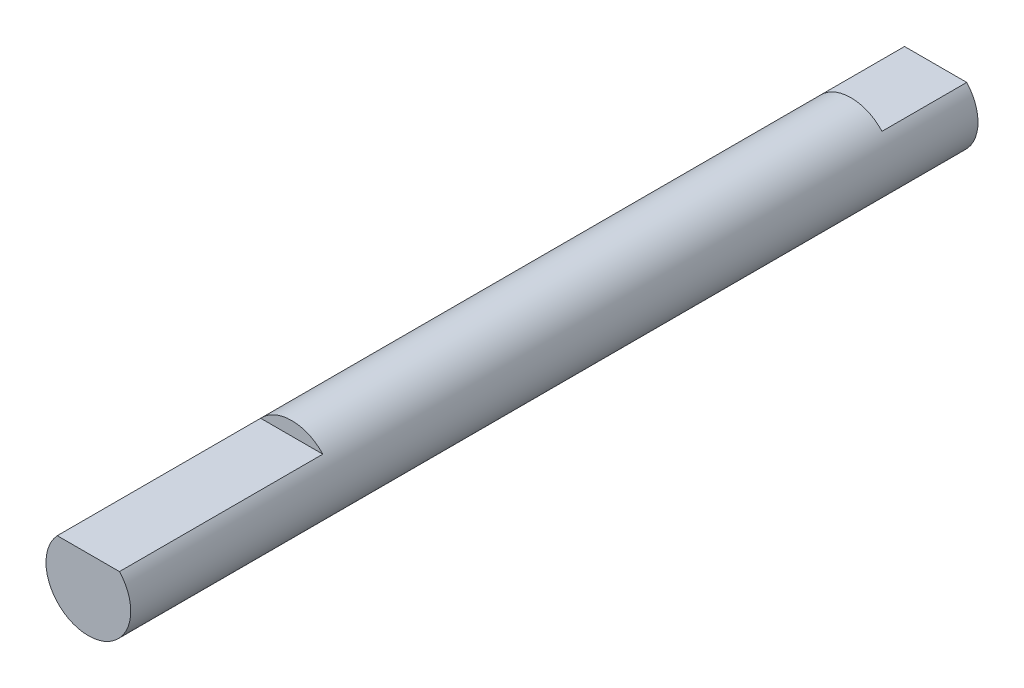
SolidWorks part; units mm, degrees
ref_plane "Front Plane" through (0, 0, 0) normal (0, 0, 1) x (1, 0, 0)
ref_plane "Top Plane" through (0, 0, 0) normal (0, 1, 0) x (1, 0, 0)
ref_plane "Right Plane" through (0, 0, 0) normal (1, 0, 0) x (0, 0, -1)
other "Configuration Table"
sketch "Sketch1" plane through (0, 0, 0) normal (0, 0, 1) x (1, 0, 0)
  circle A0 centre (0, 0) radius 2.5
  dimension "D1" = 5
extrude "Boss-Extrude1" add sketch "Sketch1" along normal blind 50
sketch "Sketch2" plane through (0, 0, 0) normal (0, 0, -1) x (-1, 0, 0)
  line L0 (-1.835, 1.6979) -> (1.835, 1.6979)
  circle A0 centre (0, 0) radius 2.5 construction
  arc A2 (1.835, 1.6979) -> (-1.835, 1.6979) centre (0, 0) ccw
  dimension "D1" = 3.67
extrude "Cut-Extrude1" cut sketch "Sketch2" against normal blind 5
sketch "Sketch3" plane through (0, 0, 50) normal (0, 0, 1) x (1, 0, 0)
  line L0 (-1.835, 1.6979) -> (1.835, 1.6979)
  circle A1 centre (0, 0) radius 2.5 construction
  arc A2 (1.835, 1.6979) -> (-1.835, 1.6979) centre (0, 0) ccw
  dimension "D1" = 3.67
extrude "Cut-Extrude3" cut sketch "Sketch3" against normal blind 12
